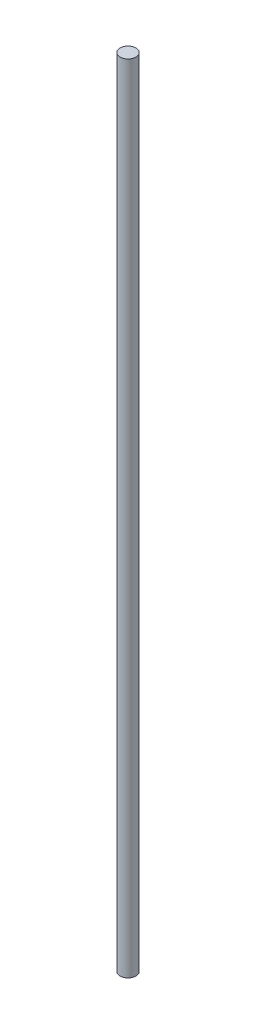
SolidWorks part; units mm, degrees
ref_plane "Front Plane" through (0, 0, 0) normal (0, 0, 1) x (1, 0, 0)
ref_plane "Top Plane" through (0, 0, 0) normal (0, 1, 0) x (1, 0, 0)
ref_plane "Right Plane" through (0, 0, 0) normal (1, 0, 0) x (0, 0, -1)
other "Configuration Table"
sketch "Sketch1" plane through (0, 0, 0) normal (0, 1, 0) x (1, 0, 0)
  circle A0 centre (0, 0) radius 10
  dimension "D1" = 20
extrude "Boss-Extrude1" add sketch "Sketch1" along normal blind 1000
